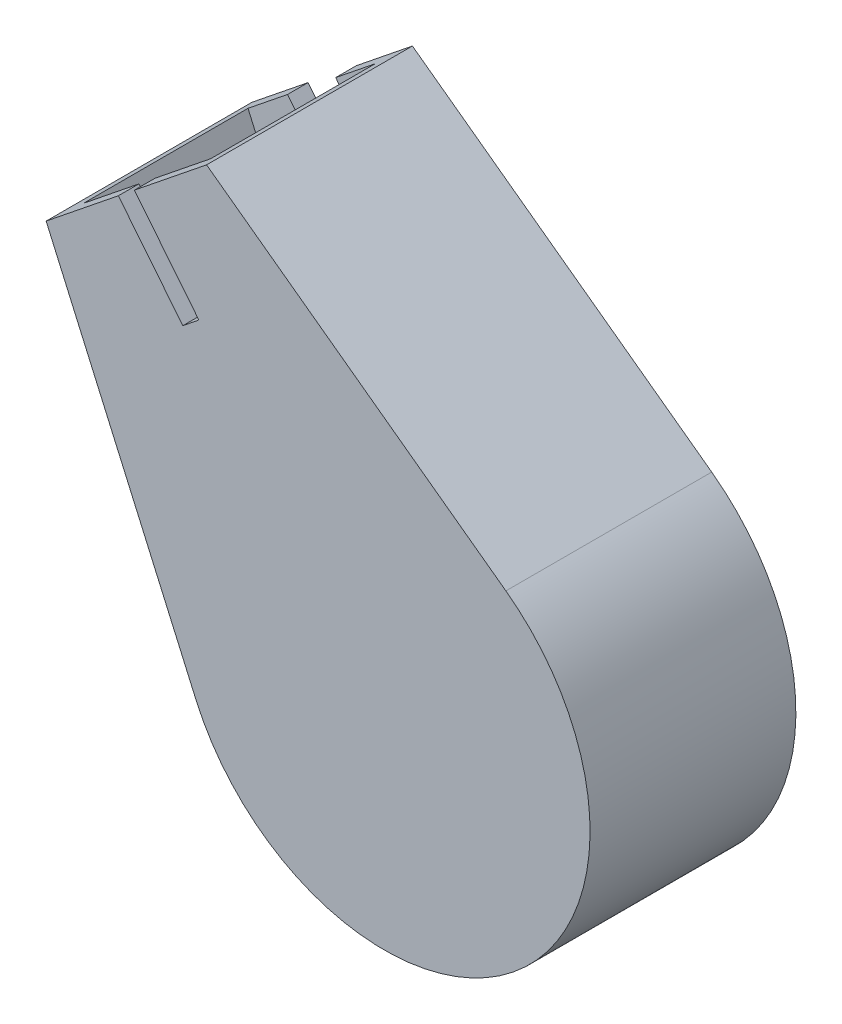
from build123d import *

# Parameters (mm, degrees)
BOSS_EXTRUDE1_DEPTH = 20
SHELL1_T            = -2
CUT_EXTRUDE1_REACH  = 55.677
CUT_EXTRUDE2_REACH  = 55.677


with BuildPart() as part:
    # Sketch1 → Boss-Extrude1 (new body)
    with BuildSketch(Plane.XY):
        with BuildLine():
            Line((-32.851981106, 24.914801572), (-18.2983008, -8.072929322))
            ThreePointArc((-18.2983008, -8.072929322), (12.528602689, -15.589551458), (11.821088788, 16.132633383))
            Line((11.821088788, 16.132633383), (-17.262429648, 37.443404261))
            Line((-17.262429648, 37.443404261), (-32.851981106, 24.914801572))
        make_face()
    extrude(amount=BOSS_EXTRUDE1_DEPTH)

    # Shell1
    shell1_openings = [part.faces().sort_by_distance(p)[0] for p in [
        (-25.057205377, 31.179102917, 10),
    ]]
    offset(amount=SHELL1_T, openings=shell1_openings, kind=Kind.INTERSECTION)

    # Sketch2 → Cut-Extrude1 (cut, up to next)
    with BuildSketch(Plane(origin=(0, 0, 0), x_dir=(-1, 0, 0), z_dir=(0, 0, -1)), mode=Mode.PRIVATE) as cut_extrude1_sk1:
        Polygon((21.131336752, 21.505036784), (16.454471314, 25.263617591), (28.983074003, 40.853169049), (33.65993944, 37.094588242), align=None)
    cut_extrude1_tool1 = extrude(cut_extrude1_sk1.sketch, amount=-CUT_EXTRUDE1_REACH, mode=Mode.PRIVATE) & part.part
    add(cut_extrude1_tool1.solids().sort_by_distance((-25.057205, 31.179103, 0))[0], mode=Mode.SUBTRACT)

    # Sketch3 → Cut-Extrude2 (cut, up to next)
    with BuildSketch(Plane.XY.offset(20), mode=Mode.PRIVATE) as cut_extrude2_sk1:
        Polygon((-18.011864488, 24.008813734), (-512.566768876, 639.391815534), (-514.125724022, 638.138955265), (-19.570819634, 22.755953465), align=None)
    cut_extrude2_tool1 = extrude(cut_extrude2_sk1.sketch, amount=-CUT_EXTRUDE2_REACH, mode=Mode.PRIVATE) & part.part
    add(cut_extrude2_tool1.solids().sort_by_distance((-266.068794, 331.073884, 20))[0], mode=Mode.SUBTRACT)


solid = part.part
